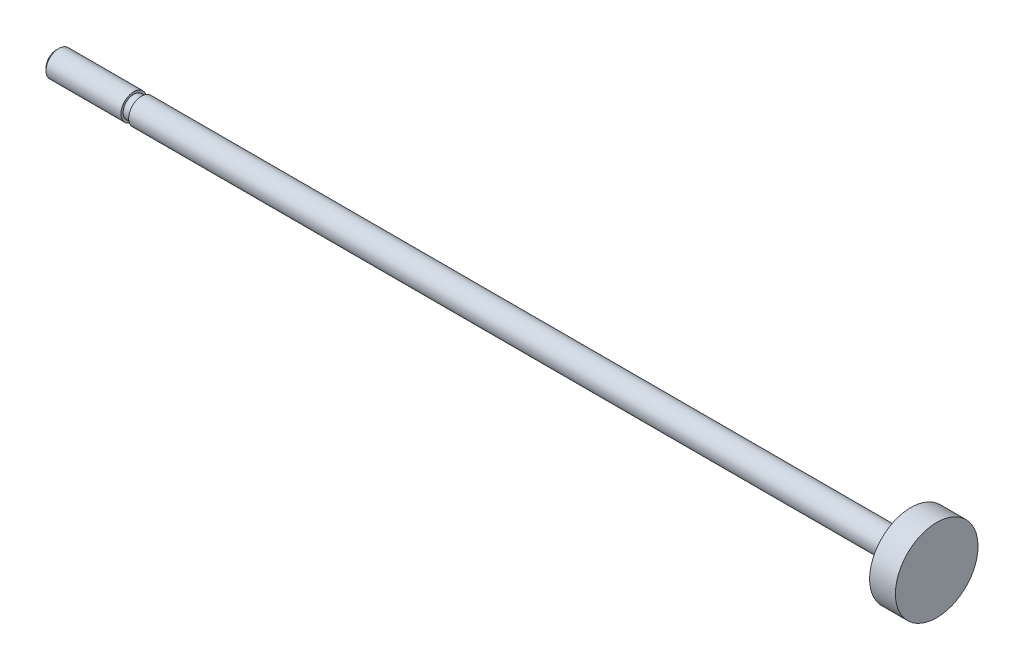
from build123d import *


with BuildPart() as part:
    # Sketch1 → Revolve1 (revolve)
    with BuildSketch(Plane.XY, mode=Mode.PRIVATE) as revolve1_sk:
        Polygon((0, 0), (0, 2.0095), (0.4905, 2.5), (15, 2.5), (15, 2.067), (16.5, 2.067), (16.5, 2.5), (165.5, 2.5), (165.5, 8), (170.5, 8), (170.5, 0), align=None)
    revolve(revolve1_sk.sketch.rotate(Axis((170.5, 0, 0), (-1, 0, 0)), 180), axis=Axis((170.5, 0, 0), (-1, 0, 0)))


solid = part.part
